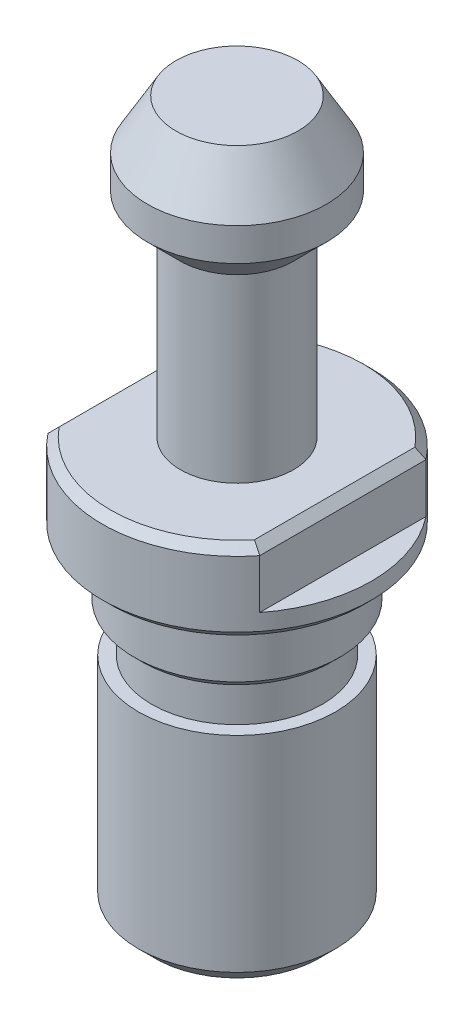
from build123d import *

# Parameters (mm, degrees)
CHAMFER_1_SIZE      = 1
SKETCH_2_W          = 3.929205492
SKETCH_2_H          = 14.159135618
CUT_EXTRUDE_1_DEPTH = 3.5
CHAMFER_2_SIZE      = 0.5


with BuildPart() as part:
    # 草图1 → 旋转1 (revolve)
    with BuildSketch(Plane.XY, mode=Mode.PRIVATE) as revolve_1_sk:
        Polygon((0, 43), (3.717949192, 43), (5.45, 40), (5.45, 38), (3.45, 36), (3.45, 25), (8.2, 25), (8.2, 20), (6.25, 20), (6.25, 16), (5.2, 16), (5.2, 13.5), (6, 13.5), (6, 0), (0, 0), align=None)
    revolve(revolve_1_sk.sketch.rotate(Axis((0, 0, 0), (0, 1, 0)), 90), axis=Axis((0, 0, 0), (0, 1, 0)))

    # 倒角1
    chamfer_1_edges = [part.edges().sort_by_distance(p)[0] for p in [
        (0, 0, 6),
    ]]
    chamfer(chamfer_1_edges, length=CHAMFER_1_SIZE)

    # 草图2 → 切除-拉伸1 (cut)
    with BuildSketch(Plane(origin=(0, 25, 0), x_dir=(1, 0, 0), z_dir=(0, 1, 0))):
        with Locations((-8.414602746, 0)):
            Rectangle(SKETCH_2_W, SKETCH_2_H)
        with Locations((8.414602746, 0)):
            Rectangle(SKETCH_2_W, SKETCH_2_H)
    extrude(amount=-CUT_EXTRUDE_1_DEPTH, mode=Mode.SUBTRACT)

    # 倒角2
    chamfer_2_edges = [part.edges().sort_by_distance(p)[0] for p in [
        (0, 16, 6.25),
        (0, 20, 8.2),
        (0, 25, 8.2),
        (3.58612191, 25, -7.374261295),
        (-6.45, 25, 0),
        (6.45, 25, 0),
    ]]
    chamfer(chamfer_2_edges, length=CHAMFER_2_SIZE)


solid = part.part
